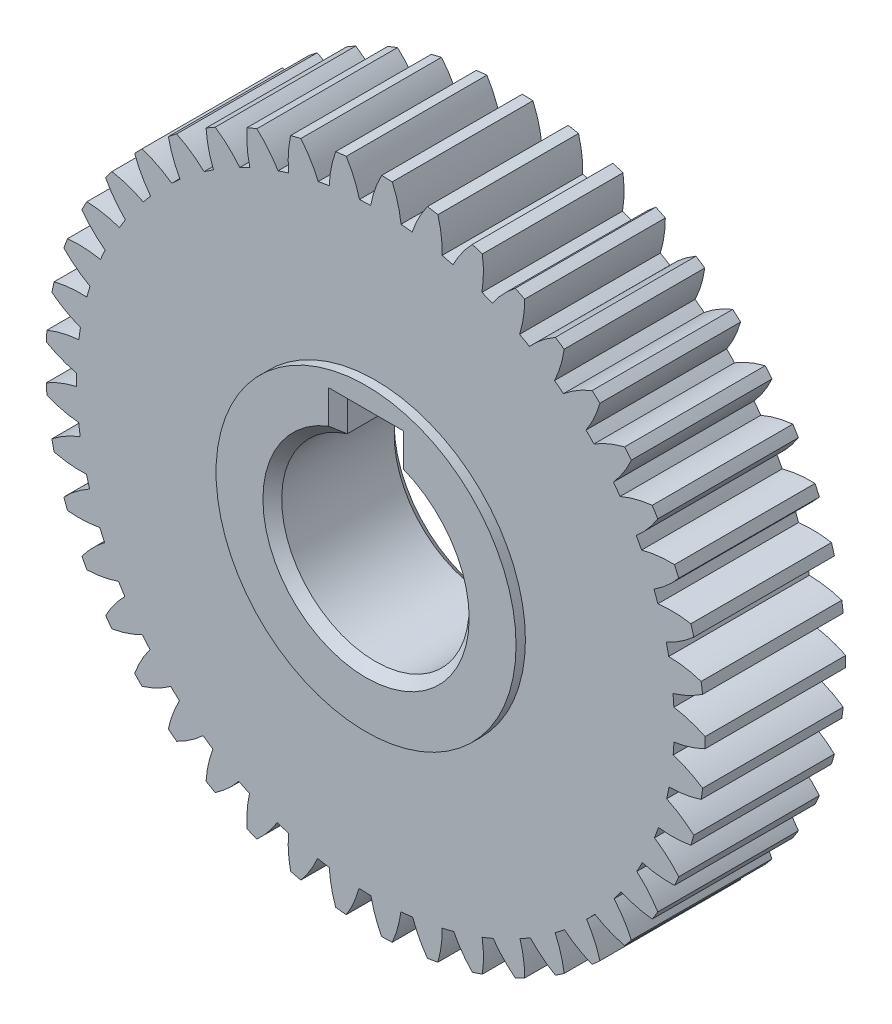
SolidWorks part; units mm, degrees
ref_plane "Front Plane" through (0, 0, 0) normal (0, 0, 1) x (1, 0, 0)
ref_plane "Top Plane" through (0, 0, 0) normal (0, 1, 0) x (1, 0, 0)
ref_plane "Right Plane" through (0, 0, 0) normal (1, 0, 0) x (0, 0, -1)
other "Configuration Table"
sketch "Sketch1" plane through (0, 0, 0) normal (0, 0, 1) x (1, 0, 0)
  circle A0 centre (0, 0) radius 31.875
  dimension "D1" = 63.75
extrude "Boss-Extrude1" add sketch "Sketch1" along normal blind 15
sketch "Sketch2" plane through (0, 0, 15) normal (0, 0, 1) x (1, 0, 0)
  line L0 (0, 0) -> (0, 35.25) construction
  line L1 (0, 0) -> (12.0562, 33.1242) construction
  line L2 (0, 0) -> (1.2302, 35.2285) construction
  line L3 (0, 33.75) -> (10.847, 29.802) construction
  circle A0 centre (0, 0) radius 33.75 construction
  circle A1 centre (0, 0) radius 35.25
  arc A2 (0.667, 35.2437) -> (-0.5092, 31.8709) centre (10.847, 29.802) ccw
  circle A3 centre (0, 0) radius 31.875 construction
  circle A4 centre (0, 0) radius 31.875
  arc A5 (1.7931, 35.2044) -> (2.7312, 31.7578) centre (-8.7417, 30.4861) cw
  dimension "D1" = 67.5
  dimension "D2" = 70.5
  dimension "D3" = 20
  dimension "D4" = 2
extrude "Boss-Extrude2" add sketch "Sketch2" against normal blind 15 contours A5 A1 A2 A4
pattern_circular "CirPattern1" count 45 over 360 about axis through (0.0029, 0.0835, 0) along (0, 0, 1) of "Boss-Extrude2"
sketch "Sketch3" plane through (0, 0, 15) normal (0, 0, 1) x (1, 0, 0)
  circle A0 centre (0, 0) radius 16
  dimension "D1" = 32
extrude "Boss-Extrude3" add sketch "Sketch3" along normal blind 1
sketch "Sketch5" plane through (0, 0, 16) normal (0, 0, 1) x (1, 0, 0)
  line L1 (-3, 7.2) -> (3, 7.2)
  line L2 (-3, 7.2) -> (-3, 12.8)
  line L3 (-3, 12.8) -> (3, 12.8)
  line L4 (3, 7.2) -> (3, 12.8)
  line L5 (-3, 7.2) -> (3, 12.8) construction
  line L6 (-3, 12.8) -> (3, 7.2) construction
  circle A0 centre (0, 0) radius 10
  point P3 (0, 10)
  dimension "D1" = 20
  dimension "D2" = 12.8
  dimension "D3" = 6
extrude "Cut-Extrude1" cut sketch "Sketch5" against normal through all contours L2 L3 L4 L1 | A0
sketch "Sketch6" plane through (0, 0, 0) normal (0, 0, -1) x (-1, 0, 0)
  circle A0 centre (0, 0) radius 20
  dimension "D1" = 40
extrude "Cut-Extrude2" cut sketch "Sketch6" against normal blind 2
chamfer "Chamfer1" distance 1 angle 45 8 edges at (-3, 11.1697, 16) (0, 12.8, 16) (3, 11.1697, 16) (0, -10, 16) (-3, 11.1697, 2) (0, 12.8, 2) (3, 11.1697, 2) (0, -10, 2)
